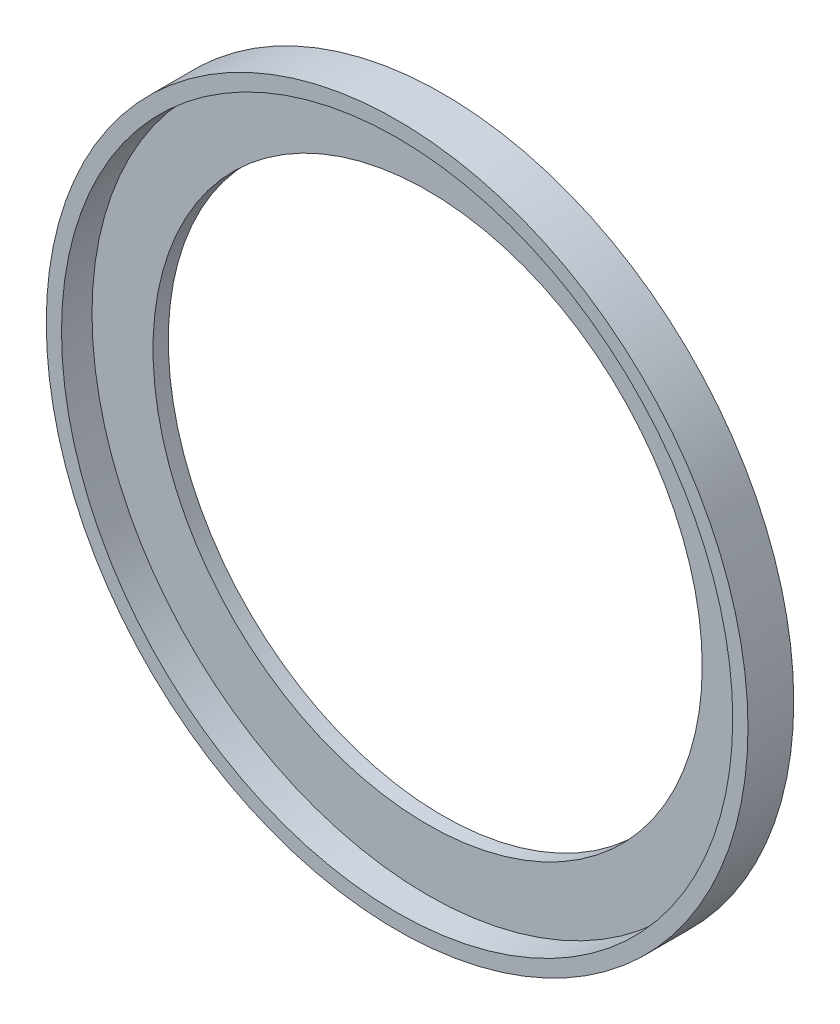
from build123d import *

# Parameters (mm, degrees)
SKETCH_1_R          = 105
EXTRUDE_1_DEPTH     = 30
SKETCH_2_R          = 90
CUT_EXTRUDE_1_DEPTH = 73
SKETCH_3_R          = 100
SKETCH_3_R_2        = 90
CUT_EXTRUDE_2_DEPTH = 25
SKETCH_4_R          = 115
SKETCH_4_R_2        = 110
EXTRUDE_2_DEPTH     = 30
SKETCH_5_R          = 105
SKETCH_5_R_2        = 100
CUT_EXTRUDE_3_DEPTH = 25
SKETCH_6_R          = 110
SKETCH_6_R_2        = 105
EXTRUDE_3_DEPTH     = 5
SKETCH_7_R          = 125
CUT_EXTRUDE_5_DEPTH = 15


with BuildPart() as part:
    # 草图1 → 凸台-拉伸1 (new body)
    with BuildSketch(Plane.XY):
        Circle(SKETCH_1_R)
    extrude(amount=EXTRUDE_1_DEPTH)

    # 草图2 → 切除-拉伸1 (cut)
    with BuildSketch(Plane.XY.offset(30)):
        Circle(SKETCH_2_R)
    extrude(amount=-CUT_EXTRUDE_1_DEPTH, mode=Mode.SUBTRACT)

    # 草图3 → 切除-拉伸2 (cut)
    with BuildSketch(Plane.XY.offset(30)):
        Circle(SKETCH_3_R)
        Circle(SKETCH_3_R_2, mode=Mode.SUBTRACT)
    extrude(amount=-CUT_EXTRUDE_2_DEPTH, mode=Mode.SUBTRACT)

    # 草图5 → 切除-拉伸3 (cut)
    with BuildSketch(Plane.XY.offset(30)):
        Circle(SKETCH_5_R)
        Circle(SKETCH_5_R_2, mode=Mode.SUBTRACT)
    extrude(amount=-CUT_EXTRUDE_3_DEPTH, mode=Mode.SUBTRACT)



with BuildPart() as body_2:
    # 草图4 → 凸台-拉伸2 (new body)
    with BuildSketch(Plane.XY.offset(30)):
        Circle(SKETCH_4_R)
        Circle(SKETCH_4_R_2, mode=Mode.SUBTRACT)
    extrude(amount=-EXTRUDE_2_DEPTH)


with BuildPart() as part_1:
    add(part.part)

    add(body_2.part)  # 凸台-拉伸3 merges body 2
    # 草图6 → 凸台-拉伸3 (add)
    with BuildSketch(Plane(origin=(0, 0, 0), x_dir=(-1, 0, 0), z_dir=(0, 0, -1))):
        with Locations(Location((0, 0, 0), (0, 0, 180))):
            Circle(SKETCH_6_R)
        Circle(SKETCH_6_R_2, mode=Mode.SUBTRACT)
    extrude(amount=-EXTRUDE_3_DEPTH)

    # 草图7 → 切除-拉伸5 (cut)
    with BuildSketch(Plane.XY.offset(30)):
        Circle(SKETCH_7_R)
    extrude(amount=-CUT_EXTRUDE_5_DEPTH, mode=Mode.SUBTRACT)


solid = part_1.part
